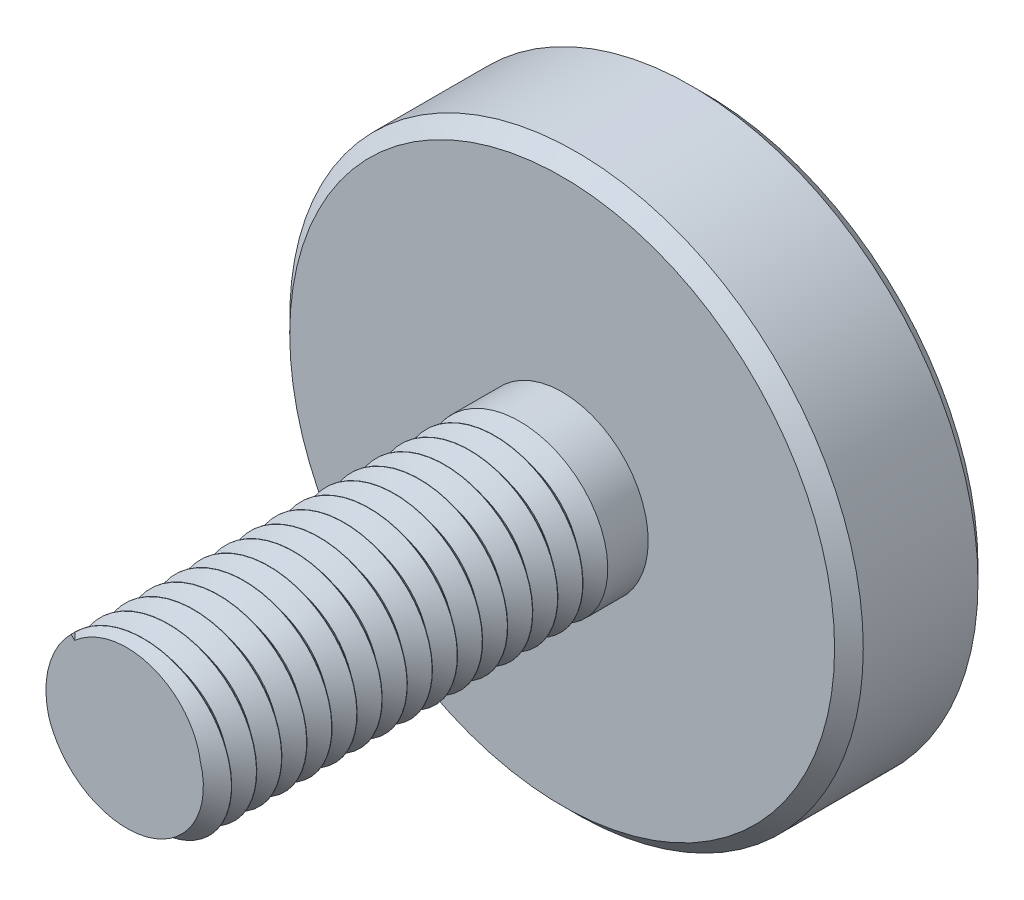
SolidWorks part; units mm, degrees
ref_plane "前视基准面" through (0, 0, 0) normal (0, 0, 1) x (1, 0, 0)
ref_plane "上视基准面" through (0, 0, 0) normal (0, 1, 0) x (1, 0, 0)
ref_plane "右视基准面" through (0, 0, 0) normal (1, 0, 0) x (0, 0, -1)
sketch "草图1" plane through (0, 0, 0) normal (0, 0, 1) x (1, 0, 0)
  circle A0 centre (0, 0) radius 20
  dimension "D1" = 40
extrude "凸台-拉伸1" add sketch "草图1" along normal blind 10
sketch "草图2" plane through (0, 0, 10) normal (0, 0, 1) x (1, 0, 0)
  circle A0 centre (0, 0) radius 6
  dimension "D1" = 12
extrude "凸台-拉伸3" add sketch "草图2" along normal blind 30
sketch "草图4" plane through (0, 0, 40) normal (0, 0, 1) x (1, 0, 0)
  circle A0 centre (0, 0) radius 6
curve "螺旋线/涡状线1" pitch 1.75 height 28 turns 16
sketch "草图5" plane through (0, 0, 0) normal (1, 0, 0) x (0, 0, -1)
  line L0 (-39.5983, 6.1414) -> (-37.6525, 6.1414)
  line L1 (-37.6525, 6.1414) -> (-38.6254, 4.8837)
  line L2 (-38.6254, 4.8837) -> (-39.5983, 6.1414)
sweep "切除-扫描1" cut profiles "草图5" path "螺旋线/涡状线1"
chamfer "倒角1" distance 1 angle 45 2 edges at (20, 0, 0) (20, 0, 10)
